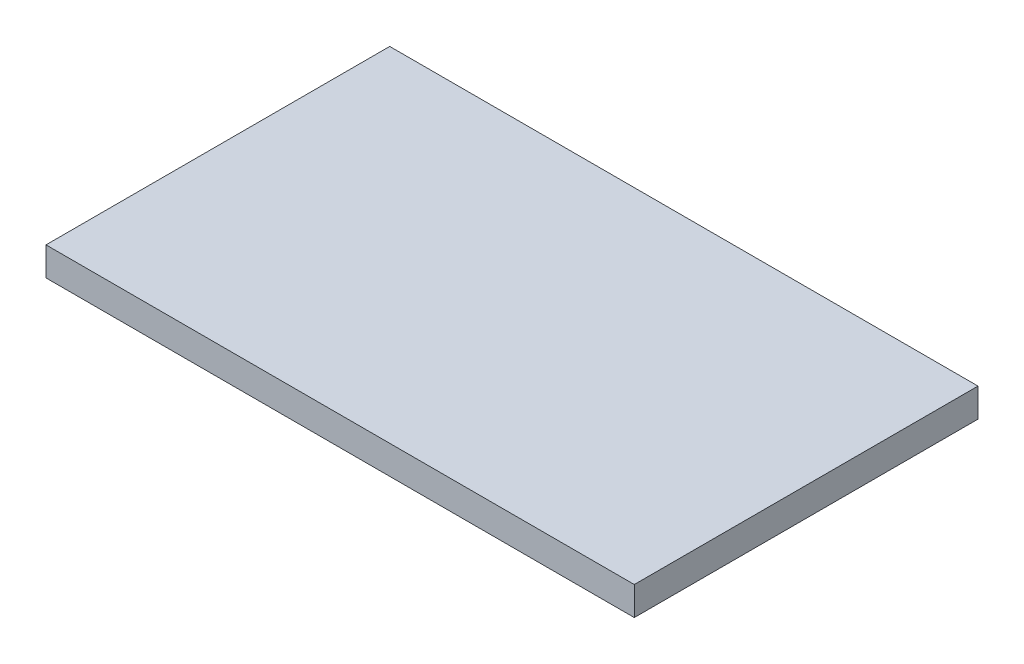
SolidWorks part; units mm, degrees
ref_plane "Front Plane" through (0, 0, 0) normal (0, 0, 1) x (1, 0, 0)
ref_plane "Top Plane" through (0, 0, 0) normal (0, 1, 0) x (1, 0, 0)
ref_plane "Right Plane" through (0, 0, 0) normal (1, 0, 0) x (0, 0, -1)
sketch "Sketch1" plane through (0, 0, 0) normal (0, 1, 0) x (1, 0, 0)
  line L0 (205.3921, 120) -> (205.3921, 0)
  line L1 (0, 0) -> (200, 0)
  line L2 (0, 0) -> (0, 120)
  line L3 (0, 120) -> (200, 120)
  line L4 (205.3921, 0) -> (200, 0)
  line L5 (205.3921, 120) -> (200, 120)
  dimension "D1" = 200
  dimension "D2" = 120
extrude "Boss-Extrude1" add sketch "Sketch1" along normal blind 10
